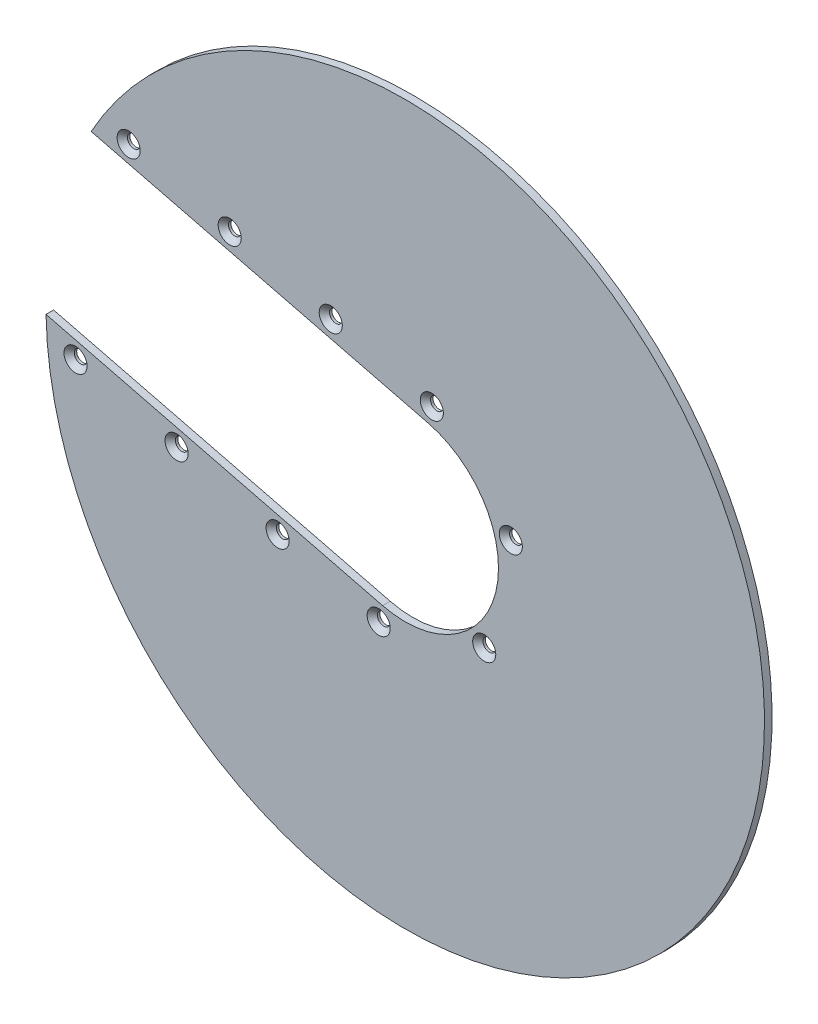
from build123d import *

# Parameters (mm, degrees)
BOSS_EXTRUDE1_DEPTH                        = 8
HOLE_SIZE_PER_FOR_TYPE_1_HEX_SOCK_2_COUNT  = 2
HOLE_SIZE_PER_FOR_TYPE_1_HEX_SOCK_2_PITCH  = 110
HOLE_SIZE_PER_FOR_TYPE_1_HEX_SOCK_3_COUNT  = 2
HOLE_SIZE_PER_FOR_TYPE_1_HEX_SOCK_3_PITCH  = 220
HOLE_SIZE_PER_FOR_TYPE_1_HEX_SOCK_4_COUNT  = 2
HOLE_SIZE_PER_FOR_TYPE_1_HEX_SOCK_4_PITCH  = 330
HOLE_SIZE_PER_FOR_TYPE_1_HEX_SOCK_5_COUNT  = 2
HOLE_SIZE_PER_FOR_TYPE_1_HEX_SOCK_5_PITCH  = 434.348828609
HOLE_SIZE_PER_FOR_TYPE_1_HEX_SOCK_6_COUNT  = 2
HOLE_SIZE_PER_FOR_TYPE_1_HEX_SOCK_6_PITCH  = 464.296139241
HOLE_SIZE_PER_FOR_TYPE_1_HEX_SOCK_7_COUNT  = 2
HOLE_SIZE_PER_FOR_TYPE_1_HEX_SOCK_7_PITCH  = 403.390629539
HOLE_SIZE_PER_FOR_TYPE_1_HEX_SOCK_8_COUNT  = 2
HOLE_SIZE_PER_FOR_TYPE_1_HEX_SOCK_8_PITCH  = 319.724881734
HOLE_SIZE_PER_FOR_TYPE_1_HEX_SOCK_9_COUNT  = 2
HOLE_SIZE_PER_FOR_TYPE_1_HEX_SOCK_9_PITCH  = 256.756694168
HOLE_SIZE_PER_FOR_TYPE_1_HEX_SOCK_10_COUNT = 2
HOLE_SIZE_PER_FOR_TYPE_1_HEX_SOCK_10_PITCH = 232


with BuildPart() as part:
    # Sketch1 → Boss-Extrude1 (new body)
    with BuildSketch(Plane.XY):
        with BuildLine():
            Line((23.829306717, 95.574129038), (-331.778451057, 184.237101079))
            ThreePointArc((-331.778451057, 184.237101079), (368.227228122, -91.80935938), (-379.43706449, -6.911156997))
            Line((-379.43706449, -6.911156997), (-23.829306717, -95.574129038))
            ThreePointArc((-23.829306717, -95.574129038), (95.574129038, -23.829306717), (23.829306717, 95.574129038))
        make_face()
    extrude(amount=BOSS_EXTRUDE1_DEPTH)

    # Sketch6 → Hole size (per %) for Type 1 hex socket Torx semi-countersunk screw (revolve, cut)
    with BuildSketch(Plane(origin=(-292.134649782, 192.388529796, 8), x_dir=(0, -1, 0), z_dir=(1, 0, 0))):
        Polygon((0, 0), (0, 8), (6.75, 8), (6.75, 5.45), (12.2, 0), align=None)
    hole_size_per_for_type_1_hex_socket_t = revolve(axis=Axis((-292.134649782, 192.388529796, 14.35), (0, 0, -1)), mode=Mode.SUBTRACT)

    # Hole size _per _ for Type 1 hex sock 2: Hole size (per %) for Type 1 hex socket Torx semi-countersunk screw ×2
    with Locations(*[Vector(0.9702957262760132, -0.24192189559960064, 0) * (i * HOLE_SIZE_PER_FOR_TYPE_1_HEX_SOCK_2_PITCH) for i in range(1, HOLE_SIZE_PER_FOR_TYPE_1_HEX_SOCK_2_COUNT)]):
        add(hole_size_per_for_type_1_hex_socket_t, mode=Mode.SUBTRACT)

    # Hole size _per _ for Type 1 hex sock 3: Hole size (per %) for Type 1 hex socket Torx semi-countersunk screw ×2
    with Locations(*[Vector(0.9702957262760132, -0.24192189559960078, 0) * (i * HOLE_SIZE_PER_FOR_TYPE_1_HEX_SOCK_3_PITCH) for i in range(1, HOLE_SIZE_PER_FOR_TYPE_1_HEX_SOCK_3_COUNT)]):
        add(hole_size_per_for_type_1_hex_socket_t, mode=Mode.SUBTRACT)

    # Hole size _per _ for Type 1 hex sock 4: Hole size (per %) for Type 1 hex socket Torx semi-countersunk screw ×2
    with Locations(*[Vector(0.9702957262760132, -0.24192189559960064, 0) * (i * HOLE_SIZE_PER_FOR_TYPE_1_HEX_SOCK_4_PITCH) for i in range(1, HOLE_SIZE_PER_FOR_TYPE_1_HEX_SOCK_4_COUNT)]):
        add(hole_size_per_for_type_1_hex_socket_t, mode=Mode.SUBTRACT)

    # Hole size _per _ for Type 1 hex sock 5: Hole size (per %) for Type 1 hex socket Torx semi-countersunk screw ×2
    with Locations(*[Vector(0.9293014736642066, -0.36932204245825073, 0) * (i * HOLE_SIZE_PER_FOR_TYPE_1_HEX_SOCK_5_PITCH) for i in range(1, HOLE_SIZE_PER_FOR_TYPE_1_HEX_SOCK_5_COUNT)]):
        add(hole_size_per_for_type_1_hex_socket_t, mode=Mode.SUBTRACT)

    # Hole size _per _ for Type 1 hex sock 6: Hole size (per %) for Type 1 hex socket Torx semi-countersunk screw ×2
    with Locations(*[Vector(0.8089192109912862, -0.587919816037217, 0) * (i * HOLE_SIZE_PER_FOR_TYPE_1_HEX_SOCK_6_PITCH) for i in range(1, HOLE_SIZE_PER_FOR_TYPE_1_HEX_SOCK_6_COUNT)]):
        add(hole_size_per_for_type_1_hex_socket_t, mode=Mode.SUBTRACT)

    # Hole size _per _ for Type 1 hex sock 7: Hole size (per %) for Type 1 hex socket Torx semi-countersunk screw ×2
    with Locations(*[Vector(0.6546302530469048, -0.7559492256730906, 0) * (i * HOLE_SIZE_PER_FOR_TYPE_1_HEX_SOCK_7_PITCH) for i in range(1, HOLE_SIZE_PER_FOR_TYPE_1_HEX_SOCK_7_COUNT)]):
        add(hole_size_per_for_type_1_hex_socket_t, mode=Mode.SUBTRACT)

    # Hole size _per _ for Type 1 hex sock 8: Hole size (per %) for Type 1 hex socket Torx semi-countersunk screw ×2
    with Locations(*[Vector(0.49210802471224957, -0.8705341417852651, 0) * (i * HOLE_SIZE_PER_FOR_TYPE_1_HEX_SOCK_8_PITCH) for i in range(1, HOLE_SIZE_PER_FOR_TYPE_1_HEX_SOCK_8_COUNT)]):
        add(hole_size_per_for_type_1_hex_socket_t, mode=Mode.SUBTRACT)

    # Hole size _per _ for Type 1 hex sock 9: Hole size (per %) for Type 1 hex socket Torx semi-countersunk screw ×2
    with Locations(*[Vector(0.19709963269028047, -0.9803834631374382, 0) * (i * HOLE_SIZE_PER_FOR_TYPE_1_HEX_SOCK_9_PITCH) for i in range(1, HOLE_SIZE_PER_FOR_TYPE_1_HEX_SOCK_9_COUNT)]):
        add(hole_size_per_for_type_1_hex_socket_t, mode=Mode.SUBTRACT)

    # Hole size _per _ for Type 1 hex sock 10: Hole size (per %) for Type 1 hex socket Torx semi-countersunk screw ×2
    with Locations(*[Vector(-0.24192189559966096, -0.9702957262759981, 0) * (i * HOLE_SIZE_PER_FOR_TYPE_1_HEX_SOCK_10_PITCH) for i in range(1, HOLE_SIZE_PER_FOR_TYPE_1_HEX_SOCK_10_COUNT)]):
        add(hole_size_per_for_type_1_hex_socket_t, mode=Mode.SUBTRACT)


solid = part.part
